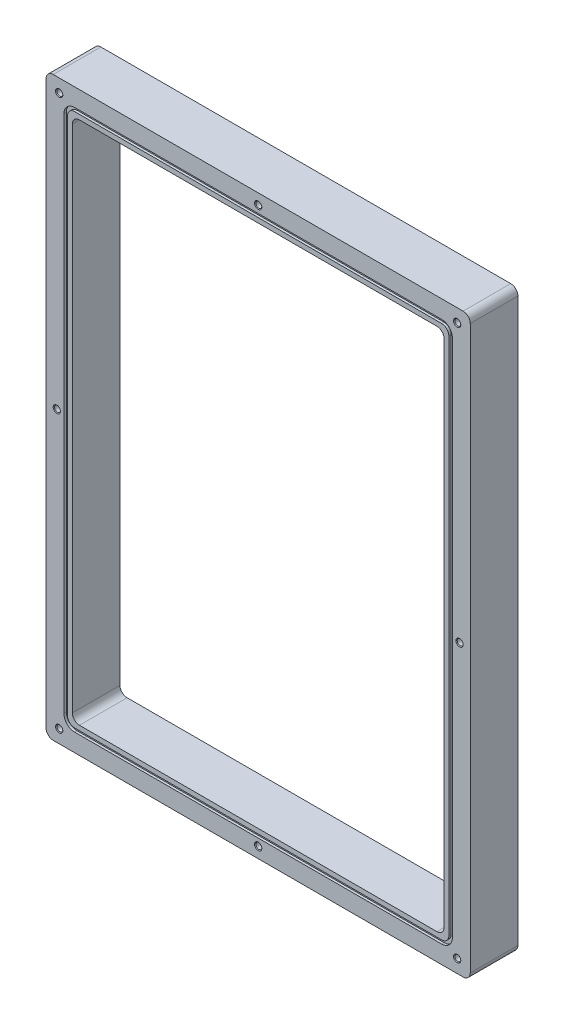
from build123d import *

# Parameters (mm, degrees)
SKETCH1_W                   = 178
SKETCH1_H                   = 242
SKETCH1_W_2                 = 156
SKETCH1_H_2                 = 220
BOSS_EXTRUDE1_DEPTH         = 20
FILLET1_R                   = 3
CUT_EXTRUDE1_DEPTH          = 1
M3_TAPPED_HOLE2_D           = 2.5
M3_TAPPED_HOLE2_DEPTH       = 6.5
M3_TAPPED_HOLE2_CSINK_D     = 3.05
M3_TAPPED_HOLE2_CSINK_ANGLE = 90
M3_TAPPED_HOLE2_TIP         = 0.751075774
M3_TAPPED_HOLE1_D           = 2.5
M3_TAPPED_HOLE1_DEPTH       = 6.5
M3_TAPPED_HOLE1_CSINK_D     = 3.05
M3_TAPPED_HOLE1_CSINK_ANGLE = 90
M3_TAPPED_HOLE1_TIP         = 0.751075774
CUT_EXTRUDE2_DEPTH          = 1


with BuildPart() as part:
    # Sketch1 → Boss-Extrude1 (new body)
    with BuildSketch(Plane.XY):
        Rectangle(SKETCH1_W, SKETCH1_H)
        Rectangle(SKETCH1_W_2, SKETCH1_H_2, mode=Mode.SUBTRACT)
    extrude(amount=BOSS_EXTRUDE1_DEPTH)

    # Fillet1
    fillet1_edges = [part.edges().sort_by_distance(p)[0] for p in [
        (78, -110, 10),
        (78, 110, 10),
        (-78, 110, 10),
        (-78, -110, 10),
        (89, 121, 10),
        (89, -121, 10),
        (-89, -121, 10),
        (-89, 121, 10),
    ]]
    fillet(fillet1_edges, radius=FILLET1_R)

    # Sketch2 → Cut-Extrude1 (cut)
    with BuildSketch(Plane.XY.offset(20)):
        with BuildLine():
            Line((-81.5, 109), (-81.5, -109))
            ThreePointArc((-81.5, -109), (-80.181980515, -112.181980515), (-77, -113.5))
            Line((-77, -113.5), (77, -113.5))
            ThreePointArc((77, -113.5), (80.181980515, -112.181980515), (81.5, -109))
            Line((81.5, -109), (81.5, 109))
            ThreePointArc((81.5, 109), (80.181980515, 112.181980515), (77, 113.5))
            Line((77, 113.5), (-77, 113.5))
            ThreePointArc((-77, 113.5), (-80.181980515, 112.181980515), (-81.5, 109))
        make_face()
        with BuildLine():
            Line((-77, -112), (77, -112))
            ThreePointArc((77, -112), (79.121320344, -111.121320344), (80, -109))
            Line((80, -109), (80, 109))
            ThreePointArc((80, 109), (79.121320344, 111.121320344), (77, 112))
            Line((77, 112), (-77, 112))
            ThreePointArc((-77, 112), (-79.121320344, 111.121320344), (-80, 109))
            Line((-80, 109), (-80, -109))
            ThreePointArc((-80, -109), (-79.121320344, -111.121320344), (-77, -112))
        make_face(mode=Mode.SUBTRACT)
    extrude(amount=-CUT_EXTRUDE1_DEPTH, mode=Mode.SUBTRACT)

    # M3 Tapped Hole2
    with Locations(Plane.XY.offset(20)):
        with Locations((-83.5, 115.5), (0, 116.5), (83.5, 115.5), (-84.5, 0.09226209), (84.5, -0.23435851), (0, -116.5), (-83.5, -115.5), (83.5, -115.5)):
            CounterSinkHole(M3_TAPPED_HOLE2_D / 2, M3_TAPPED_HOLE2_CSINK_D / 2, depth=M3_TAPPED_HOLE2_DEPTH, counter_sink_angle=M3_TAPPED_HOLE2_CSINK_ANGLE)
            with Locations((0, 0, -(M3_TAPPED_HOLE2_DEPTH + M3_TAPPED_HOLE2_TIP / 2))):  # 118° drill point
                Cone(0, M3_TAPPED_HOLE2_D / 2, M3_TAPPED_HOLE2_TIP, mode=Mode.SUBTRACT)

    # M3 Tapped Hole1
    with Locations(Plane(origin=(0, 0, 0), x_dir=(-1, 0, 0), z_dir=(0, 0, -1))):
        with Locations((0, 113), (-81, 0), (81, 0), (0, -113), (80, -112), (-80, -112), (-80, 112), (80, 112)):
            CounterSinkHole(M3_TAPPED_HOLE1_D / 2, M3_TAPPED_HOLE1_CSINK_D / 2, depth=M3_TAPPED_HOLE1_DEPTH, counter_sink_angle=M3_TAPPED_HOLE1_CSINK_ANGLE)
            with Locations((0, 0, -(M3_TAPPED_HOLE1_DEPTH + M3_TAPPED_HOLE1_TIP / 2))):  # 118° drill point
                Cone(0, M3_TAPPED_HOLE1_D / 2, M3_TAPPED_HOLE1_TIP, mode=Mode.SUBTRACT)

    # Sketch5 → Cut-Extrude2 (cut)
    with BuildSketch(Plane(origin=(0, 0, 0), x_dir=(-1, 0, 0), z_dir=(0, 0, -1))):
        with BuildLine():
            Line((-81.5, -118), (81.5, -118))
            ThreePointArc((81.5, -118), (84.681980515, -116.681980515), (86, -113.5))
            Line((86, -113.5), (86, 113.5))
            ThreePointArc((86, 113.5), (84.681980515, 116.681980515), (81.5, 118))
            Line((81.5, 118), (-81.5, 118))
            ThreePointArc((-81.5, 118), (-84.681980515, 116.681980515), (-86, 113.5))
            Line((-86, 113.5), (-86, -113.5))
            ThreePointArc((-86, -113.5), (-84.681980515, -116.681980515), (-81.5, -118))
        make_face()
        with BuildLine():
            Line((-84.5, 113.5), (-84.5, -113.5))
            ThreePointArc((-84.5, -113.5), (-83.621320344, -115.621320344), (-81.5, -116.5))
            Line((-81.5, -116.5), (81.5, -116.5))
            ThreePointArc((81.5, -116.5), (83.621320344, -115.621320344), (84.5, -113.5))
            Line((84.5, -113.5), (84.5, 113.5))
            ThreePointArc((84.5, 113.5), (83.621320344, 115.621320344), (81.5, 116.5))
            Line((81.5, 116.5), (-81.5, 116.5))
            ThreePointArc((-81.5, 116.5), (-83.621320344, 115.621320344), (-84.5, 113.5))
        make_face(mode=Mode.SUBTRACT)
    extrude(amount=-CUT_EXTRUDE2_DEPTH, mode=Mode.SUBTRACT)


solid = part.part
